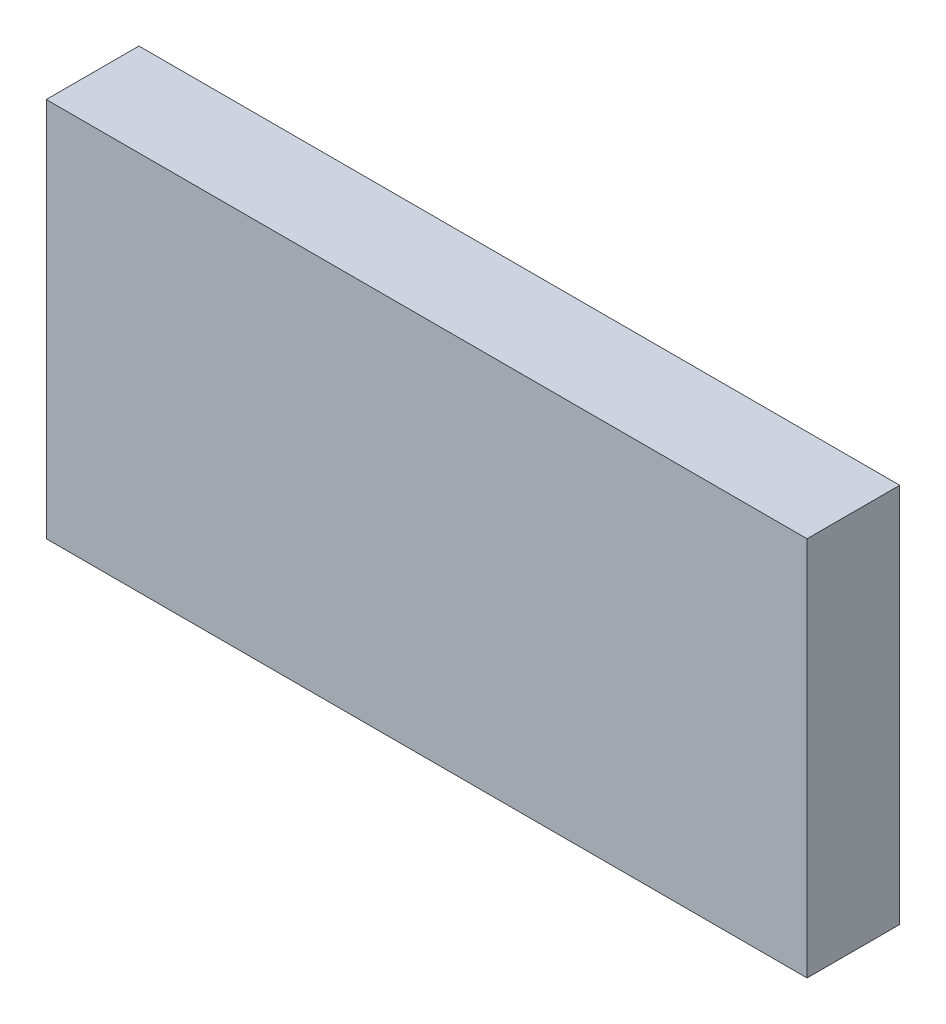
SolidWorks part; units mm, degrees
ref_plane "Front Plane" through (0, 0, 0) normal (0, 0, 1) x (1, 0, 0)
ref_plane "Top Plane" through (0, 0, 0) normal (0, 1, 0) x (1, 0, 0)
ref_plane "Right Plane" through (0, 0, 0) normal (1, 0, 0) x (0, 0, -1)
sketch "Sketch1" plane through (0, 0, 0) normal (0, 1, 0) x (1, 0, 0)
  line L1 (-195, 23.75) -> (195, 23.75)
  line L2 (-195, 23.75) -> (-195, -23.75)
  line L3 (-195, -23.75) -> (195, -23.75)
  line L4 (195, 23.75) -> (195, -23.75)
  line L5 (-195, 23.75) -> (195, -23.75) construction
  line L6 (-195, -23.75) -> (195, 23.75) construction
  point P0 (0, 0)
  dimension "D1" = 390
  dimension "D2" = 47.5
extrude "Boss-Extrude1" add sketch "Sketch1" along normal blind 195
shell "Shell1" thickness 6
